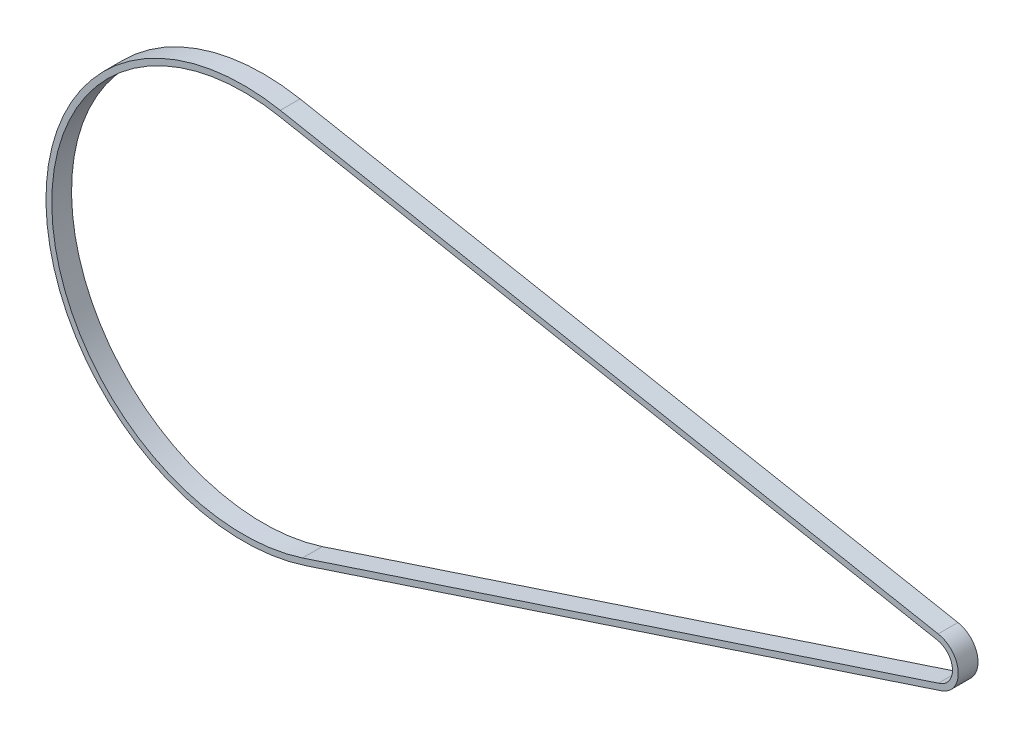
from build123d import *

# Parameters (mm, degrees)
SKETCH2_W = 20
SKETCH2_H = 6


with BuildPart() as part:
    # Sweep1: sweep along a path in Sketch1
    with BuildLine(Plane.XY) as sweep1_path:
        Line((-803.471602915, -72.580053696), (-137.514764545, -198.618968438))
        ThreePointArc((-137.514764545, -198.618968438), (-117.217555143, -221.543328014), (-134.339730828, -246.927064367))
        Line((-134.339730828, -246.927064367), (-778.071333179, -459.044821132))
        ThreePointArc((-778.071333179, -459.044821132), (-1040.232770199, -282.208199453), (-803.471602915, -72.580053696))
    # Sketch2 → Sweep1 (sweep)
    with BuildSketch(Plane(origin=(-803.471602915, 0, 0), x_dir=(0, 0, -1), z_dir=(1, 0, 0))):
        with Locations((0, -75.580053696)):
            Rectangle(SKETCH2_W, SKETCH2_H)
    sweep(path=sweep1_path.line)


solid = part.part
